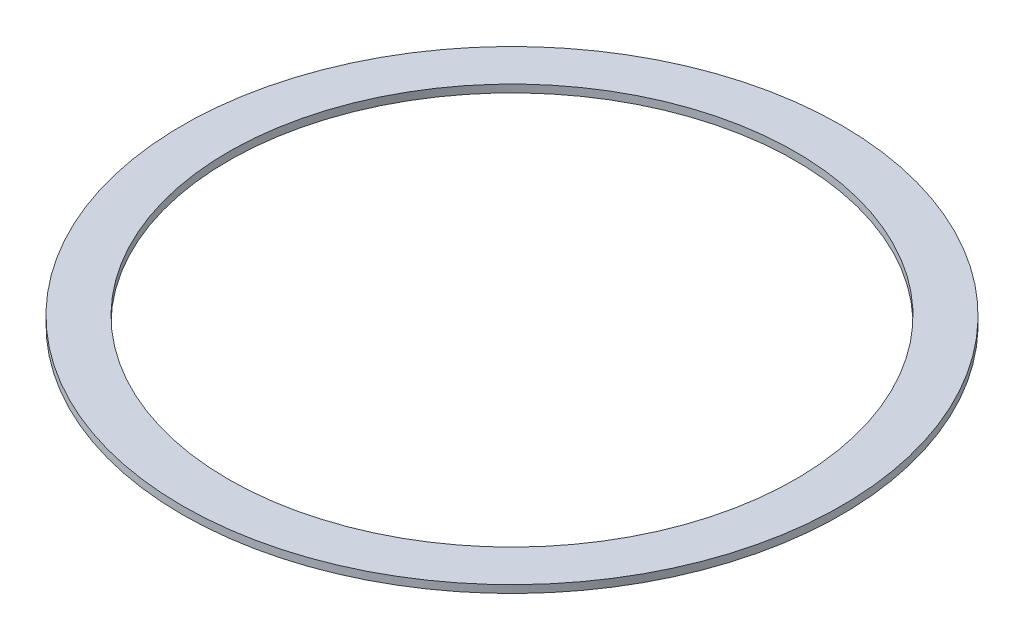
SolidWorks part; units mm, degrees
material "C (石墨)"
ref_plane "Front Plane" through (0, 0, 0) normal (0, 0, 1) x (1, 0, 0)
ref_plane "Top Plane" through (0, 0, 0) normal (0, 1, 0) x (1, 0, 0)
ref_plane "Right Plane" through (0, 0, 0) normal (1, 0, 0) x (0, 0, -1)
sketch "Sketch1" plane through (0, 0, 0) normal (0, 1, 0) x (1, 0, 0)
  circle A0 centre (0, 0) radius 37
  circle A1 centre (0, 0) radius 43
  dimension "D1" = 74
  dimension "D2" = 86
extrude "Boss-Extrude1" add sketch "Sketch1" along normal blind 1
